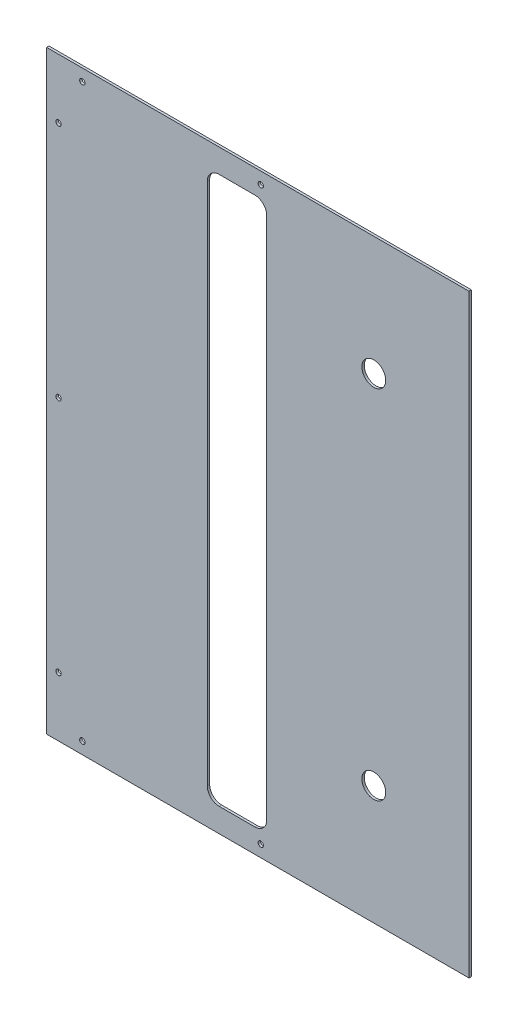
SolidWorks part; units mm, degrees
material "Q235A"
ref_plane "前视基准面" through (0, 0, 0) normal (0, 0, 1) x (1, 0, 0)
ref_plane "上视基准面" through (0, 0, 0) normal (0, 1, 0) x (1, 0, 0)
ref_plane "右视基准面" through (0, 0, 0) normal (1, 0, 0) x (0, 0, -1)
sketch "草图1" plane through (0, 0, 0) normal (0, 0, 1) x (1, 0, 0)
  line L1 (-177.5, 250) -> (177.5, 250)
  line L2 (-177.5, 250) -> (-177.5, -250)
  line L3 (-177.5, -250) -> (177.5, -250)
  line L4 (177.5, 250) -> (177.5, -250)
  line L5 (0, -250) -> (0, 250) construction
  line L6 (-177.5, 0) -> (177.5, 0) construction
  point P0 (0, 0)
  dimension "D1" = 355
  dimension "D2" = 500
extrude "凸台-拉伸1" add sketch "草图1" along normal blind 2
hole_wizard "Ø4.5 (4.5) 直径孔1" positions "草图2" profile "草图3" hole size "Ø4.5" standard "GB"
sketch "草图2" plane through (0, 0, 2) normal (0, 0, 1) x (1, 0, 0)
  line L1 (-167.5, -240) -> (32.5, -240) construction
  line L2 (-167.5, -240) -> (-167.5, 240) construction
  line L3 (-167.5, 240) -> (32.5, 240) construction
  line L4 (32.5, -240) -> (32.5, 240) construction
  line L5 (-67.5, 240) -> (-67.5, -240) construction
  line L6 (-167.5, 0) -> (32.5, 0) construction
  line L7 (-177.5, 250) -> (-177.5, -250) construction
  point P330 (-167.5, 0)
  point P336 (-167.5, 200)
  point P341 (-167.5, -200)
  point P342 (-147.5, 240)
  point P344 (2.5, 240)
  point P347 (2.5, -240)
  point P348 (-147.5, -240)
  dimension "D1" = 200
  dimension "D2" = 480
  dimension "D3" = 150
  dimension "D4" = 200
  dimension "D5" = 20
  dimension "D6" = 10
sketch "草图3" plane through (-147.5, -240, 2) normal (1, 0, 0) x (0, -1, 0)
  line L0 (0, 0) -> (0, 9.3519)
  line L1 (0, 9.3519) -> (2.25, 8)
  line L2 (2.25, 8) -> (2.25, 0)
  line L5 (2.25, 0) -> (0, 0)
  line L10 (0, 9.3519) -> (-2.25, 8) construction
  line L11 (0, -6.35) -> (0, 107.95) construction
  dimension "孔直径" = 4.5
  dimension "孔深度" = 8
  dimension "导头角度" = 118
sketch "草图4" plane through (0, 0, 0) normal (0, 0, -1) x (-1, 0, 0)
  line L0 (-177.5, 0) -> (177.5, 0) construction
  line L1 (-177.5, -250) -> (-177.5, 250) construction
  line L2 (177.5, 250) -> (177.5, -250) construction
  line L4 (-7.5, -230) -> (42.5, -230)
  line L5 (-7.5, -230) -> (-7.5, 230)
  line L6 (-7.5, 230) -> (42.5, 230)
  line L7 (42.5, -230) -> (42.5, 230)
  line L8 (17.5, 230) -> (17.5, -230) construction
  line L9 (-7.5, 0) -> (42.5, 0) construction
  point P6 (17.5, 0)
  dimension "D1" = 170
  dimension "D2" = 50
  dimension "D3" = 460
extrude "切除-拉伸1" cut sketch "草图4" against normal blind 10
fillet "圆角1" radius 10 4 edges at (-42.5, -230, 1) (7.5, -230, 1) (-42.5, 230, 1) (7.5, 230, 1)
sketch "草图5" plane through (0, 0, 0) normal (0, 0, -1) x (-1, 0, 0)
  line L0 (-177.5, 0) -> (177.5, 0) construction
  line L1 (-177.5, -250) -> (-177.5, 250) construction
  line L2 (177.5, 250) -> (177.5, -250) construction
  line L3 (-97.5, -150) -> (-97.5, 150) construction
  circle A0 centre (-97.5, -150) radius 10
  circle A1 centre (-97.5, 150) radius 10
  dimension "D3" = 20
  dimension "D1" = 80
  dimension "D2" = 300
extrude "切除-拉伸2" cut sketch "草图5" against normal blind 10
